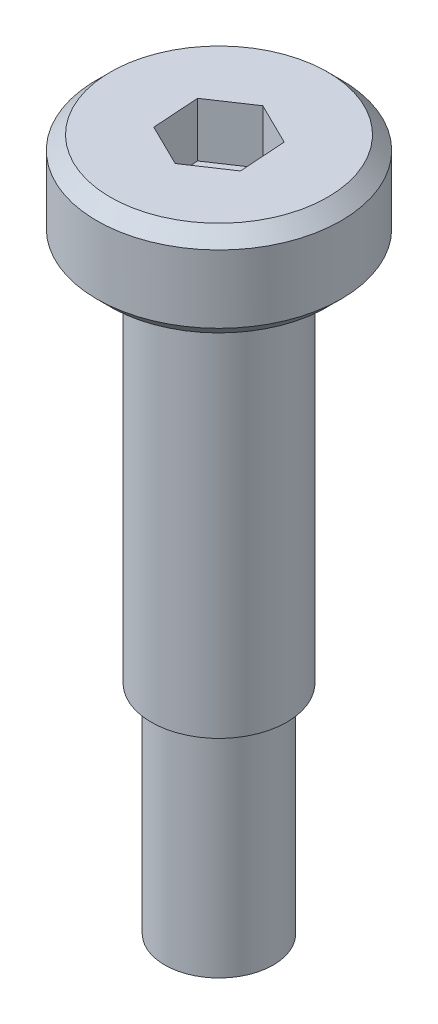
from build123d import *

# Parameters (mm, degrees)
CUT_EXTRUDE1_DEPTH = 2
CHAMFER1_SIZE      = 0.5


with BuildPart() as part:
    # Sketch1 → Revolve1 (revolve)
    with BuildSketch(Plane.XY, mode=Mode.PRIVATE) as revolve1_sk:
        Polygon((0, 0), (0, 25.5), (-4.5, 25.5), (-4.5, 22), (-2.5, 22), (-2.5, 8), (-2, 8), (-2, 0), align=None)
    revolve(revolve1_sk.sketch.rotate(Axis((0, 0, 0), (0, 1, 0)), 180), axis=Axis((0, 0, 0), (0, 1, 0)))

    # Sketch2 → Cut-Extrude1 (cut)
    with BuildSketch(Plane(origin=(0, 25.5, 0), x_dir=(1, 0, 0), z_dir=(0, 1, 0))):
        Polygon((1.554085232, -0.764734655), (1.439322254, 0.963509963), (-0.114762978, 1.728244618), (-1.554085232, 0.764734655), (-1.439322254, -0.963509963), (0.114762978, -1.728244618), align=None)
    extrude(amount=-CUT_EXTRUDE1_DEPTH, mode=Mode.SUBTRACT)

    # Chamfer1
    chamfer1_edges = [part.edges().sort_by_distance(p)[0] for p in [
        (-4.5, 22, 0),
        (-4.5, 25.5, 0),
    ]]
    chamfer(chamfer1_edges, length=CHAMFER1_SIZE)


solid = part.part
